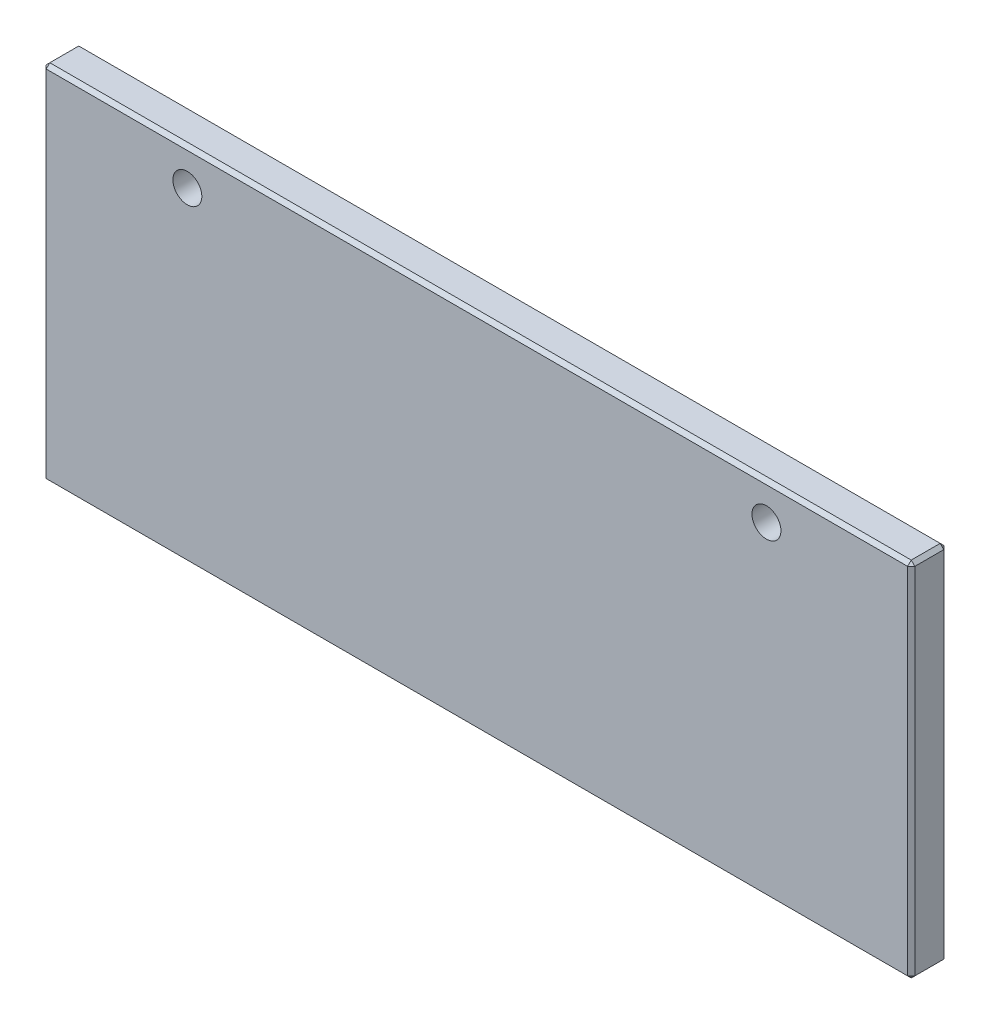
from build123d import *

# Parameters (mm, degrees)
SKETCH1_W                 = 120
SKETCH1_H                 = 50
BOSS_EXTRUDE1_DEPTH       = 5
F_4_0MM_DOWEL_HOLE1_D     = 4
F_4_0MM_DOWEL_HOLE1_DEPTH = 12
F_4_0MM_DOWEL_HOLE1_TIP   = 1.201721238
CHAMFER1_SIZE             = 0.5


with BuildPart() as part:
    # Sketch1 → Boss-Extrude1 (new body)
    with BuildSketch(Plane.XY):
        with Locations((60, 25)):
            Rectangle(SKETCH1_W, SKETCH1_H)
    extrude(amount=BOSS_EXTRUDE1_DEPTH)

    # Ø4.0mm dowel hole1
    with Locations(Plane.XY.offset(5)):
        with Locations((20, 45), (100, 45)):
            Hole(F_4_0MM_DOWEL_HOLE1_D / 2, depth=F_4_0MM_DOWEL_HOLE1_DEPTH)
            with Locations((0, 0, -(F_4_0MM_DOWEL_HOLE1_DEPTH + F_4_0MM_DOWEL_HOLE1_TIP / 2))):  # 118° drill point
                Cone(0, F_4_0MM_DOWEL_HOLE1_D / 2, F_4_0MM_DOWEL_HOLE1_TIP, mode=Mode.SUBTRACT)

    # Chamfer1
    chamfer1_edges = [part.edges().sort_by_distance(p)[0] for p in [
        (120, 25, 5),
        (60, 50, 5),
        (0, 25, 5),
        (60, 50, 0),
        (120, 25, 0),
        (60, 0, 0),
        (0, 25, 0),
        (0, 50, 2.5),
        (120, 50, 2.5),
        (120, 0, 2.5),
        (0, 0, 2.5),
        (60, 0, 5),
    ]]
    chamfer(chamfer1_edges, length=CHAMFER1_SIZE)


solid = part.part
